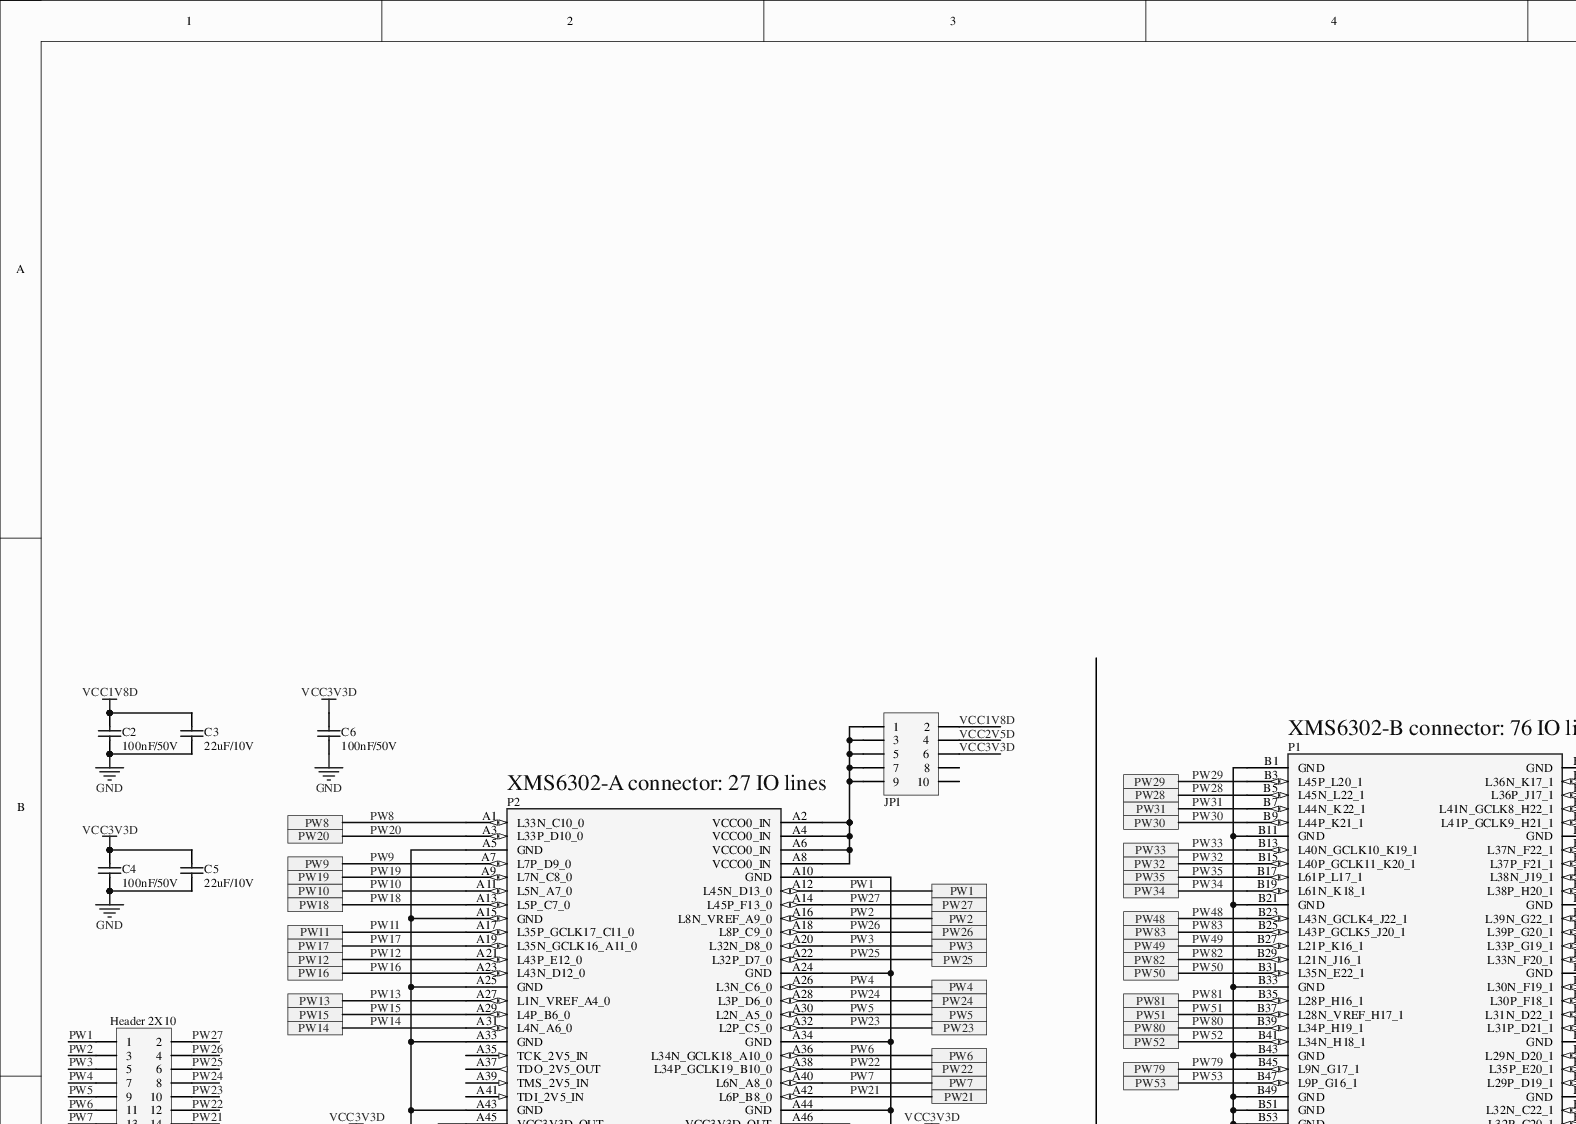
[diagram p0: MISC82195-4.SchDoc, top left]
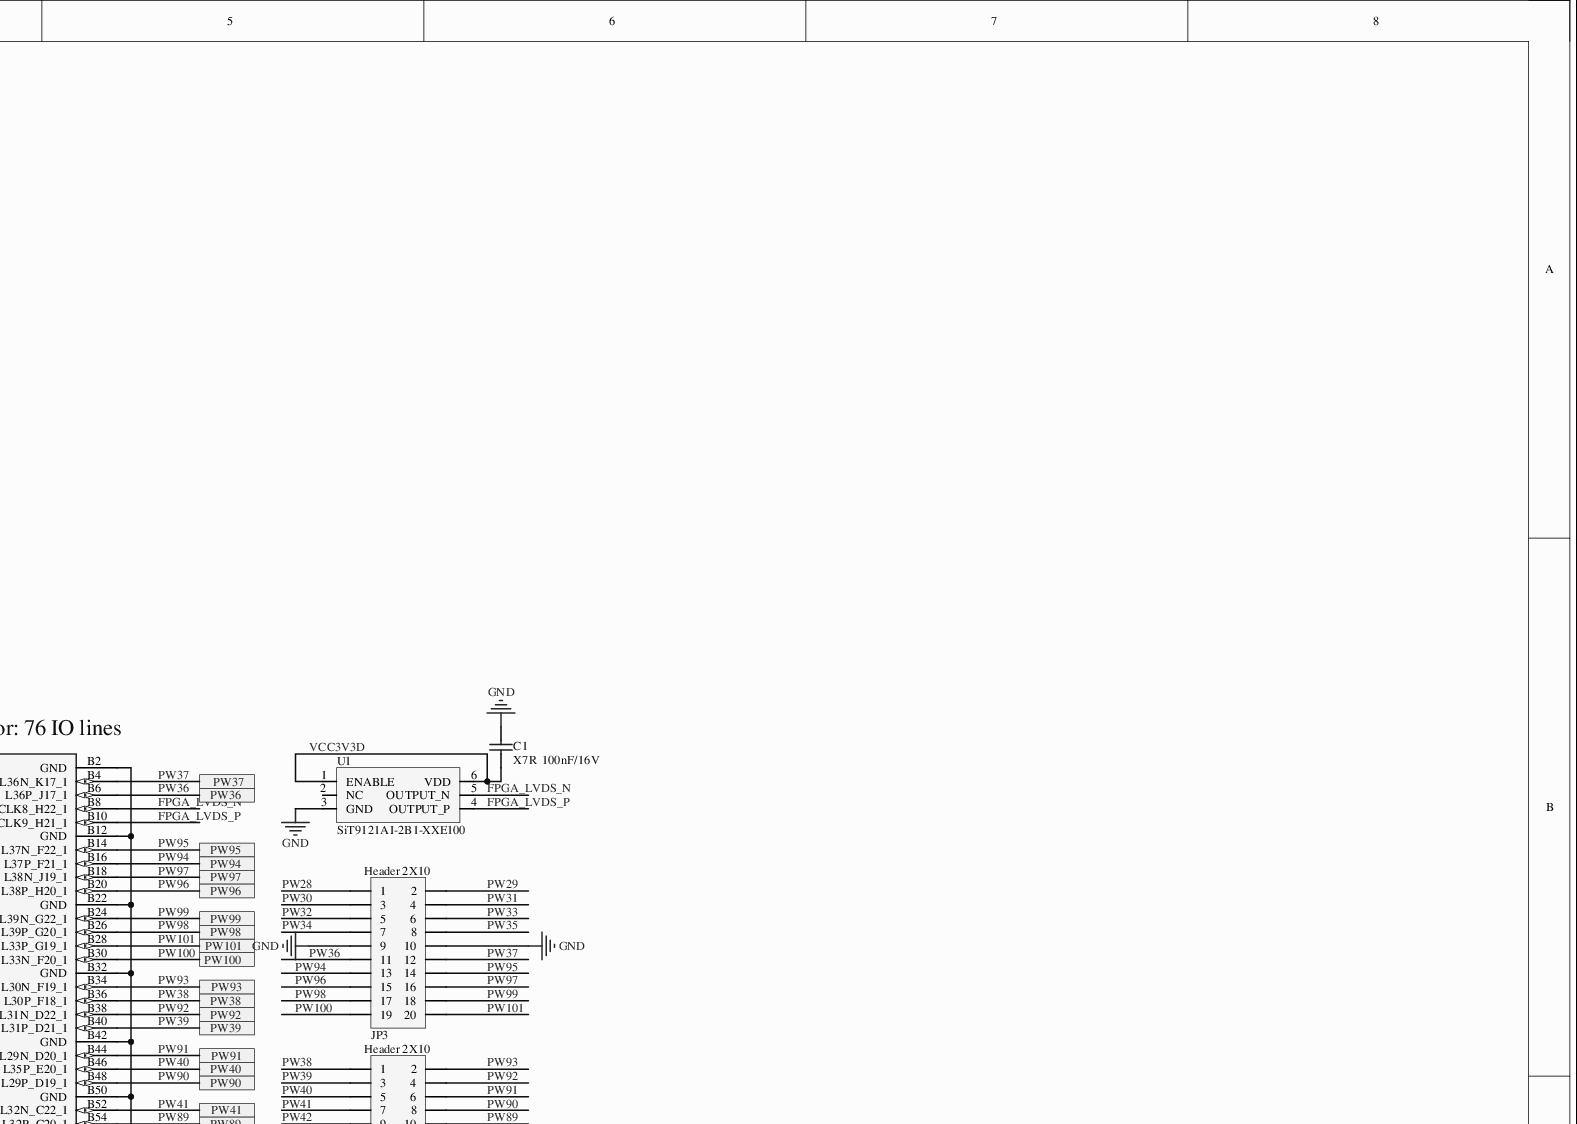
[diagram p1: MISC82195-4.SchDoc, top right]
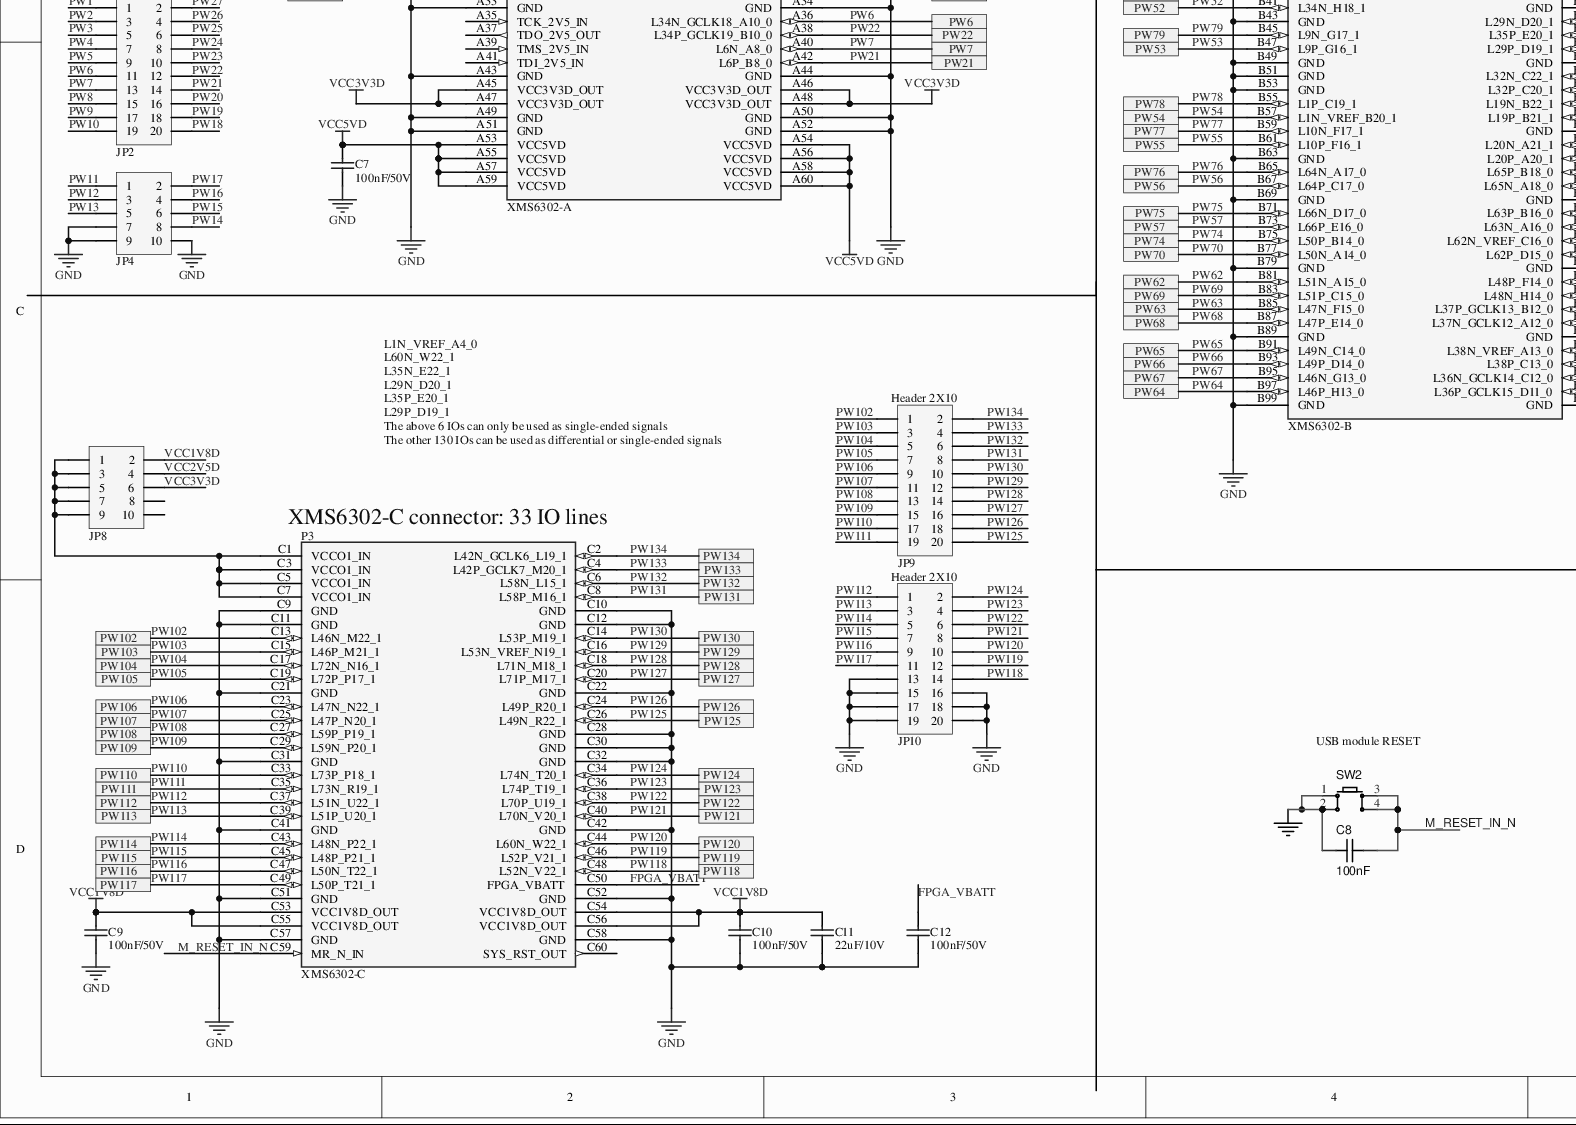
[diagram p2: MISC82195-4.SchDoc, bottom left]
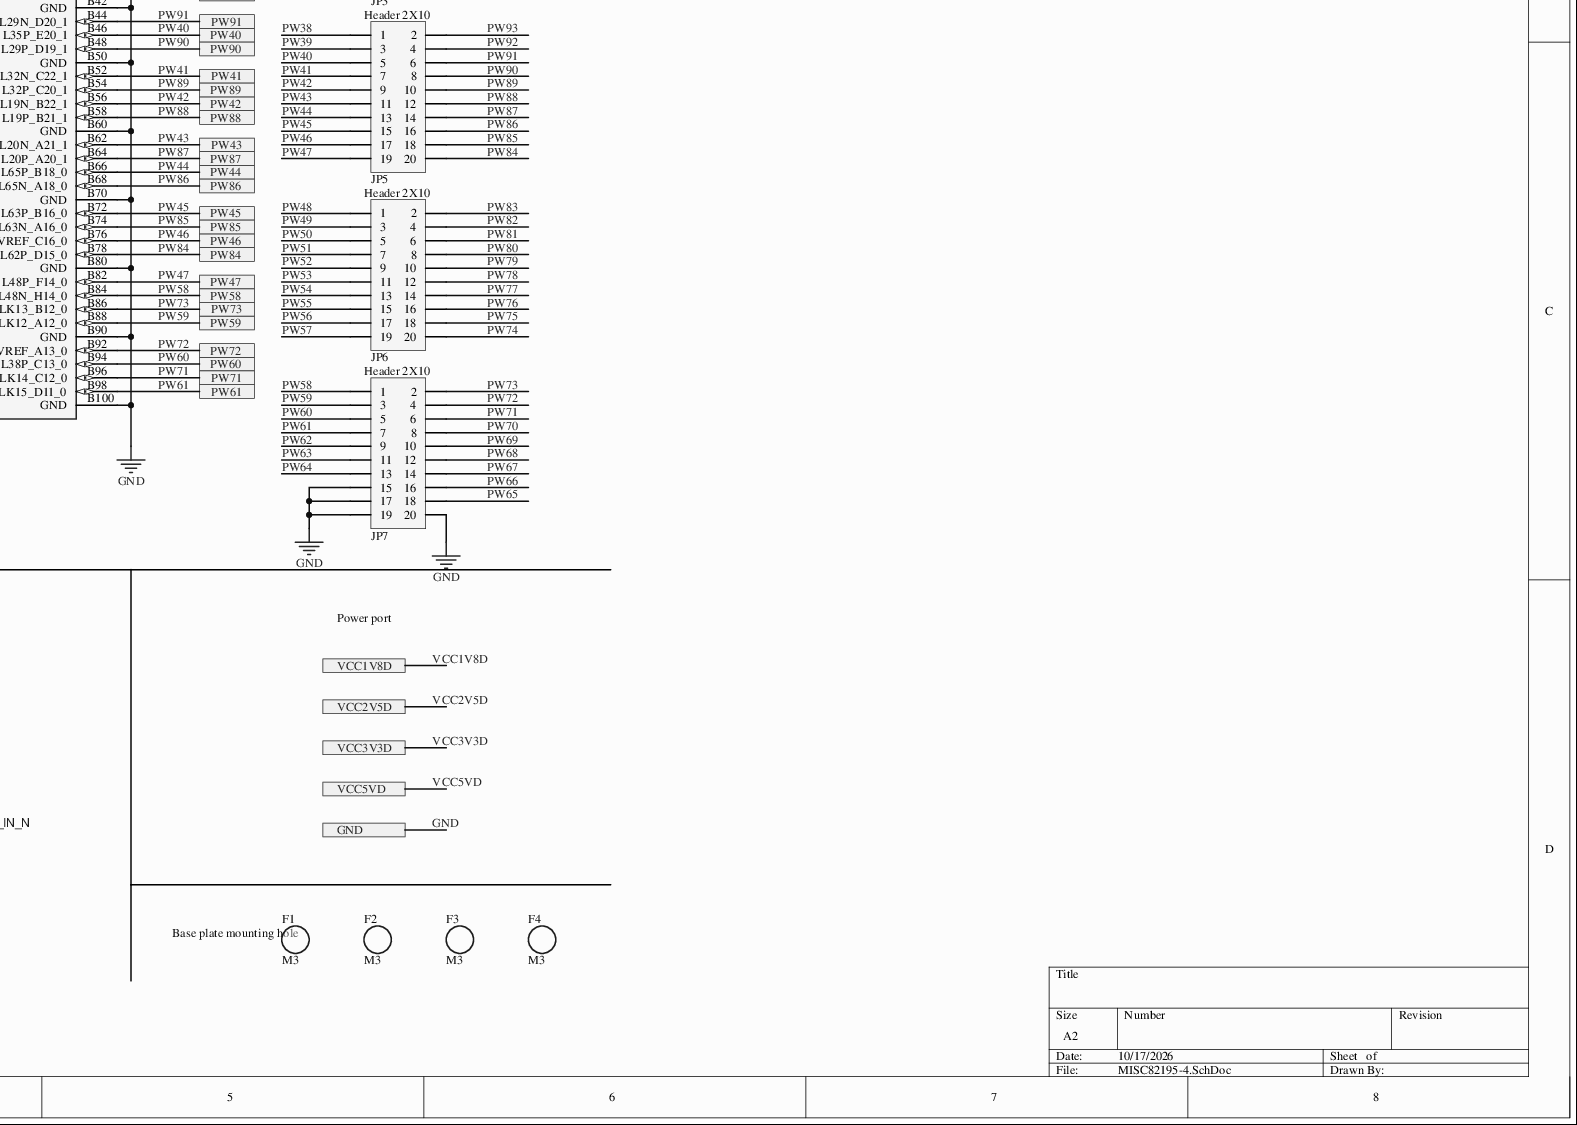
[diagram p3: MISC82195-4.SchDoc, bottom right]
# Altium project MISC82195-8.PrjPcb (part 1 of 2)
3 sheets, 214 parts. Net scope: global (net labels, ports and power ports of the same name join across sheets).
Board file: MISC82195.PcbDoc
Sheets:
  MISC82195-4.SchDoc
  MISC82195-2.SchDoc
  MISC82195-10.SchDoc

## Sheet MISC82195-4.SchDoc
size A2; SheetNumber: 1; SheetTotal: 3

### Parts
C1  X7R  100nF/16V  [C0603]
C2  100nF/50V  [C0603]
C3  22uF/10V  [C0603]
C4  100nF/50V  [C0603]
C5  22uF/10V  [C0603]
C6  100nF/50V  [C0603]
C7  100nF/50V  [C0603]
C8  100nF  [C0603]
C9  100nF/50V  [C0603]
C10  100nF/50V  [C0603]
C11  22uF/10V  [C0603]
C12  100nF/50V  [C0603]
F1  M3  [M3]
F2  M3  [M3]
F3  M3  [M3]
F4  M3  [M3]
JP1  Header 5X2  [HDR2.54-LI-2x5P]  (value not drawn)
JP2  Header 2X10  [HDR2.54-LI-2x10P]
JP3  Header 2X10  [HDR2.54-LI-2x10P]
JP4  Header 5X2  [HDR2.54-LI-2x5P]  (value not drawn)
JP5  Header 2X10  [HDR2.54-LI-2x10P]
JP6  Header 2X10  [HDR2.54-LI-2x10P]
JP7  Header 2X10  [HDR2.54-LI-2x10P]
JP8  Header 5X2  [HDR2.54-LI-2x5P]  (value not drawn)
JP9  Header 2X10  [HDR2.54-LI-2x10P]
JP10  Header 2X10  [HDR2.54-LI-2x10P]
P1  XMS6302-B  [XMS6302-B]
P2  XMS6302-A  [XMS6302-A]
P3  XMS6302-C  [XMS6302-C]
SW2  Key_SMD_6x6x6.5  [SW-SMD_4P-L6.0-W6.0-P4.50-LS9.0-2]  (value not drawn)
U1  SiT9121AI-2B1-XXE100  [3225-6p]

### Ports
GND, PW1, PW2, PW3, PW4, PW5, PW6, PW7, PW8, PW9, PW10, PW11, PW12, PW13, PW14, PW15, PW16, PW17, PW18, PW19, PW20, PW21, PW22, PW23, PW24, PW25, PW26, PW27, PW28, PW29, PW30, PW31, PW32, PW33, PW34, PW35, PW36, PW37, PW38, PW39, PW40, PW41, PW42, PW43, PW44, PW45, PW46, PW47, PW48, PW49, PW50, PW51, PW52, PW53, PW54, PW55, PW56, PW57, PW58, PW59, PW60, PW61, PW62, PW63, PW64, PW65, PW66, PW67, PW68, PW69, PW70, PW71, PW72, PW73, PW74, PW75, PW76, PW77, PW78, PW79, PW80, PW81, PW82, PW83, PW84, PW85, PW86, PW87, PW88, PW89, PW90, PW91, PW92, PW93, PW94, PW95, PW96, PW97, PW98, PW99, PW100, PW101, PW102, PW103, PW104, PW105, PW106, PW107, PW108, PW109, PW110, PW111, PW112, PW113, PW114, PW115, PW116, PW117, PW118, PW119, PW120, PW121, PW122, PW123, PW124, PW125, PW126, PW127, PW128, PW129, PW130, PW131, PW132, PW133, PW134, VCC1V8D, VCC2V5D, VCC3V3D, VCC5VD

### Nets
GND: C1.2 C2.1 C3.1 C4.1 C5.1 C6.1 C7.1 C8.2 C9.1 C10.1 C11.1 C12.2 JP3.9 JP3.10 JP4.7 JP4.9 JP4.10 JP7.15 JP7.17 JP7.19 JP7.20 JP10.13 JP10.15 JP10.16 JP10.17 JP10.18 JP10.19 JP10.20 P1.B1(GND) P1.B2(GND) P1.B11(GND) P1.B12(GND) P1.B21(GND) P1.B22(GND) P1.B32(GND) P1.B33(GND) P1.B42(GND) P1.B43(GND) P1.B49(GND) P1.B50(GND) P1.B51(GND) P1.B53(GND) P1.B60(GND) P1.B63(GND) P1.B69(GND) P1.B70(GND) P1.B79(GND) P1.B80(GND) P1.B89(GND) P1.B90(GND) P1.B99(GND) P1.B100(GND) P2.A5(GND) P2.A10(GND) P2.A15(GND) P2.A24(GND) P2.A25(GND) P2.A33(GND) P2.A34(GND) P2.A43(GND) P2.A44(GND) P2.A49(GND) P2.A50(GND) P2.A51(GND) P2.A52(GND) P3.C9(GND) P3.C10(GND) P3.C11(GND) P3.C12(GND) P3.C21(GND) P3.C22(GND) P3.C28(GND) P3.C30(GND) P3.C31(GND) P3.C32(GND) P3.C41(GND) P3.C42(GND) P3.C51(GND) P3.C52(GND) P3.C57(GND) P3.C58(GND) SW2.1 SW2.2 U1.3(GND) ; port GND
VCC1V8D: C2.2 C3.2 C9.2 C10.2 C11.2 JP1.2 JP8.2 P3.C53(VCC1V8D_OUT) P3.C54(VCC1V8D_OUT) P3.C55(VCC1V8D_OUT) P3.C56(VCC1V8D_OUT) ; port VCC1V8D
VCC3V3D: C1.1 C4.2 C5.2 C6.2 JP1.6 JP8.6 P2.A45(VCC3V3D_OUT) P2.A46(VCC3V3D_OUT) P2.A47(VCC3V3D_OUT) P2.A48(VCC3V3D_OUT) U1.1(ENABLE) U1.6(VDD) ; port VCC3V3D
VCC5VD: C7.2 P2.A53(VCC5VD) P2.A54(VCC5VD) P2.A55(VCC5VD) P2.A56(VCC5VD) P2.A57(VCC5VD) P2.A58(VCC5VD) P2.A59(VCC5VD) P2.A60(VCC5VD) ; port VCC5VD
FPGA_LVDS_N: P1.B8(L41N_GCLK8_H22_1) U1.5(OUTPUT_N)
FPGA_LVDS_P: P1.B10(L41P_GCLK9_H21_1) U1.4(OUTPUT_P)
FPGA_VBATT: C12.1 P3.C50(FPGA_VBATT)
M_RESET_IN_N: C8.1 P3.C59(MR_N_IN) SW2.3 SW2.4
PW1: JP2.1 P2.A12(L45N_D13_0) ; port PW1
PW2: JP2.3 P2.A16(L8N_VREF_A9_0) ; port PW2
PW3: JP2.5 P2.A20(L32N_D8_0) ; port PW3
PW4: JP2.7 P2.A26(L3N_C6_0) ; port PW4  [project net CS_DAC1]
PW5: JP2.9 P2.A30(L2N_A5_0) ; port PW5  [project net CS_DAC2]
PW6: JP2.11 P2.A36(L34N_GCLK18_A10_0) ; port PW6  [project net CS_DAC3]
PW7: JP2.13 P2.A40(L6N_A8_0) ; port PW7
PW8: JP2.15 P2.A1(L33N_C10_0) ; port PW8
PW9: JP2.17 P2.A7(L7P_D9_0) ; port PW9
PW10: JP2.19 P2.A11(L5N_A7_0) ; port PW10
PW11: JP4.1 P2.A17(L35P_GCLK17_C11_0) ; port PW11
PW12: JP4.3 P2.A21(L43P_E12_0) ; port PW12
PW13: JP4.5 P2.A27(L1N_VREF_A4_0) ; port PW13
PW14: JP4.8 P2.A31(L4N_A6_0) ; port PW14
PW15: JP4.6 P2.A29(L4P_B6_0) ; port PW15
PW16: JP4.4 P2.A23(L43N_D12_0) ; port PW16
PW17: JP4.2 P2.A19(L35N_GCLK16_A11_0) ; port PW17
PW18: JP2.20 P2.A13(L5P_C7_0) ; port PW18
PW19: JP2.18 P2.A9(L7N_C8_0) ; port PW19
PW20: JP2.16 P2.A3(L33P_D10_0) ; port PW20
PW21: JP2.14 P2.A42(L6P_B8_0) ; port PW21
PW22: JP2.12 P2.A38(L34P_GCLK19_B10_0) ; port PW22
PW23: JP2.10 P2.A32(L2P_C5_0) ; port PW23
PW24: JP2.8 P2.A28(L3P_D6_0) ; port PW24
PW25: JP2.6 P2.A22(L32P_D7_0) ; port PW25
PW26: JP2.4 P2.A18(L8P_C9_0) ; port PW26
PW27: JP2.2 P2.A14(L45P_F13_0) ; port PW27
PW28: JP3.1 P1.B5(L45N_L22_1) ; port PW28
PW29: JP3.2 P1.B3(L45P_L20_1) ; port PW29
PW30: JP3.3 P1.B9(L44P_K21_1) ; port PW30
PW31: JP3.4 P1.B7(L44N_K22_1) ; port PW31
PW32: JP3.5 P1.B15(L40P_GCLK11_K20_1) ; port PW32
PW33: JP3.6 P1.B13(L40N_GCLK10_K19_1) ; port PW33
PW34: JP3.7 P1.B19(L61N_K18_1) ; port PW34
PW35: JP3.8 P1.B17(L61P_L17_1) ; port PW35
PW36: JP3.11 P1.B6(L36P_J17_1) ; port PW36
PW37: JP3.12 P1.B4(L36N_K17_1) ; port PW37
PW38: JP5.1 P1.B36(L30P_F18_1) ; port PW38
PW39: JP5.3 P1.B40(L31P_D21_1) ; port PW39
PW40: JP5.5 P1.B46(L35P_E20_1) ; port PW40
PW41: JP5.7 P1.B52(L32N_C22_1) ; port PW41
PW42: JP5.9 P1.B56(L19N_B22_1) ; port PW42
PW43: JP5.11 P1.B62(L20N_A21_1) ; port PW43
PW44: JP5.13 P1.B66(L65P_B18_0) ; port PW44
PW45: JP5.15 P1.B72(L63P_B16_0) ; port PW45
PW46: JP5.17 P1.B76(L62N_VREF_C16_0) ; port PW46
PW47: JP5.19 P1.B82(L48P_F14_0) ; port PW47
PW48: JP6.1 P1.B23(L43N_GCLK4_J22_1) ; port PW48
PW49: JP6.3 P1.B27(L21P_K16_1) ; port PW49
PW50: JP6.5 P1.B31(L35N_E22_1) ; port PW50
PW51: JP6.7 P1.B37(L28N_VREF_H17_1) ; port PW51
PW52: JP6.9 P1.B41(L34N_H18_1) ; port PW52
PW53: JP6.11 P1.B47(L9P_G16_1) ; port PW53
PW54: JP6.13 P1.B57(L1N_VREF_B20_1) ; port PW54
PW55: JP6.15 P1.B61(L10P_F16_1) ; port PW55
PW56: JP6.17 P1.B67(L64P_C17_0) ; port PW56
PW57: JP6.19 P1.B73(L66P_E16_0) ; port PW57
PW58: JP7.1 P1.B84(L48N_H14_0) ; port PW58
PW59: JP7.3 P1.B88(L37N_GCLK12_A12_0) ; port PW59
PW60: JP7.5 P1.B94(L38P_C13_0) ; port PW60
PW61: JP7.7 P1.B98(L36P_GCLK15_D11_0) ; port PW61
PW62: JP7.9 P1.B81(L51N_A15_0) ; port PW62
PW63: JP7.11 P1.B85(L47N_F15_0) ; port PW63
PW64: JP7.13 P1.B97(L46P_H13_0) ; port PW64
PW65: JP7.18 P1.B91(L49N_C14_0) ; port PW65
PW66: JP7.16 P1.B93(L49P_D14_0) ; port PW66
PW67: JP7.14 P1.B95(L46N_G13_0) ; port PW67
PW68: JP7.12 P1.B87(L47P_E14_0) ; port PW68
PW69: JP7.10 P1.B83(L51P_C15_0) ; port PW69
PW70: JP7.8 P1.B77(L50N_A14_0) ; port PW70
PW71: JP7.6 P1.B96(L36N_GCLK14_C12_0) ; port PW71
PW72: JP7.4 P1.B92(L38N_VREF_A13_0) ; port PW72
PW73: JP7.2 P1.B86(L37P_GCLK13_B12_0) ; port PW73
PW74: JP6.20 P1.B75(L50P_B14_0) ; port PW74
PW75: JP6.18 P1.B71(L66N_D17_0) ; port PW75
PW76: JP6.16 P1.B65(L64N_A17_0) ; port PW76
PW77: JP6.14 P1.B59(L10N_F17_1) ; port PW77
PW78: JP6.12 P1.B55(L1P_C19_1) ; port PW78
PW79: JP6.10 P1.B45(L9N_G17_1) ; port PW79
PW80: JP6.8 P1.B39(L34P_H19_1) ; port PW80
PW81: JP6.6 P1.B35(L28P_H16_1) ; port PW81
PW82: JP6.4 P1.B29(L21N_J16_1) ; port PW82
PW83: JP6.2 P1.B25(L43P_GCLK5_J20_1) ; port PW83
PW84: JP5.20 P1.B78(L62P_D15_0) ; port PW84
PW85: JP5.18 P1.B74(L63N_A16_0) ; port PW85
PW86: JP5.16 P1.B68(L65N_A18_0) ; port PW86
PW87: JP5.14 P1.B64(L20P_A20_1) ; port PW87
PW88: JP5.12 P1.B58(L19P_B21_1) ; port PW88
PW89: JP5.10 P1.B54(L32P_C20_1) ; port PW89
PW90: JP5.8 P1.B48(L29P_D19_1) ; port PW90
PW91: JP5.6 P1.B44(L29N_D20_1) ; port PW91
PW92: JP5.4 P1.B38(L31N_D22_1) ; port PW92
PW93: JP5.2 P1.B34(L30N_F19_1) ; port PW93  [project net CS_CDAC1]
PW94: JP3.13 P1.B16(L37P_F21_1) ; port PW94
PW95: JP3.14 P1.B14(L37N_F22_1) ; port PW95
PW96: JP3.15 P1.B20(L38P_H20_1) ; port PW96
PW97: JP3.16 P1.B18(L38N_J19_1) ; port PW97
PW98: JP3.17 P1.B26(L39P_G20_1) ; port PW98
PW99: JP3.18 P1.B24(L39N_G22_1) ; port PW99
PW100: JP3.19 P1.B30(L33N_F20_1) ; port PW100
PW101: JP3.20 P1.B28(L33P_G19_1) ; port PW101
PW102: JP9.1 P3.C13(L46N_M22_1) ; port PW102
PW103: JP9.3 P3.C15(L46P_M21_1) ; port PW103
PW104: JP9.5 P3.C17(L72N_N16_1) ; port PW104
PW105: JP9.7 P3.C19(L72P_P17_1) ; port PW105
PW106: JP9.9 P3.C23(L47N_N22_1) ; port PW106
PW107: JP9.11 P3.C25(L47P_N20_1) ; port PW107
PW108: JP9.13 P3.C27(L59P_P19_1) ; port PW108
PW109: JP9.15 P3.C29(L59N_P20_1) ; port PW109
PW110: JP9.17 P3.C33(L73P_P18_1) ; port PW110
PW111: JP9.19 P3.C35(L73N_R19_1) ; port PW111
PW112: JP10.1 P3.C37(L51N_U22_1) ; port PW112
PW113: JP10.3 P3.C39(L51P_U20_1) ; port PW113
PW114: JP10.5 P3.C43(L48N_P22_1) ; port PW114
PW115: JP10.7 P3.C45(L48P_P21_1) ; port PW115
PW116: JP10.9 P3.C47(L50N_T22_1) ; port PW116
PW117: JP10.11 P3.C49(L50P_T21_1) ; port PW117
PW118: JP10.14 P3.C48(L52N_V22_1) ; port PW118
PW119: JP10.12 P3.C46(L52P_V21_1) ; port PW119
PW120: JP10.10 P3.C44(L60N_W22_1) ; port PW120
PW121: JP10.8 P3.C40(L70N_V20_1) ; port PW121
PW122: JP10.6 P3.C38(L70P_U19_1) ; port PW122
PW123: JP10.4 P3.C36(L74P_T19_1) ; port PW123
PW124: JP10.2 P3.C34(L74N_T20_1) ; port PW124
PW125: JP9.20 P3.C26(L49N_R22_1) ; port PW125
PW126: JP9.18 P3.C24(L49P_R20_1) ; port PW126
PW127: JP9.16 P3.C20(L71P_M17_1) ; port PW127
PW128: JP9.14 P3.C18(L71N_M18_1) ; port PW128
PW129: JP9.12 P3.C16(L53N_VREF_N19_1) ; port PW129
PW130: JP9.10 P3.C14(L53P_M19_1) ; port PW130
PW131: JP9.8 P3.C8(L58P_M16_1) ; port PW131
PW132: JP9.6 P3.C6(L58N_L15_1) ; port PW132
PW133: JP9.4 P3.C4(L42P_GCLK7_M20_1) ; port PW133
PW134: JP9.2 P3.C2(L42N_GCLK6_L19_1) ; port PW134
VCC2V5D: JP1.4 JP8.4 ; port VCC2V5D
NetJP1_1: JP1.1 JP1.3 JP1.5 JP1.7 JP1.9 P2.A2(VCCO0_IN) P2.A4(VCCO0_IN) P2.A6(VCCO0_IN) P2.A8(VCCO0_IN)
NetJP8_1: JP8.1 JP8.3 JP8.5 JP8.7 JP8.9 P3.C1(VCCO1_IN) P3.C3(VCCO1_IN) P3.C5(VCCO1_IN) P3.C7(VCCO1_IN)

Not connected (* = marked no-connect by the designer): JP1 8 10; JP8 8 10; P2 A35(TCK_2V5_IN) A37(TDO_2V5_OUT) A39(TMS_2V5_IN) A41(TDI_2V5_IN); P3 C60(SYS_RST_OUT); U1 2(NC)

### Notes on the sheet
- (near P1) XMS6302-B connector: 76 IO lines
- XMS6302-A connector: 27 IO lines
- L1N_VREF_A4_0
- L60N_W22_1
- L35N_E22_1
- L29N_D20_1
- L35P_E20_1
- L29P_D19_1
- The above 6 IOs can only be used as single-ended signals
- The other 130 IOs can be used as differential or single-ended signals
- (near P3) XMS6302-C connector: 33 IO lines
- Power port
- (near SW2) USB module RESET
- (near F1) Base plate mounting hole

### Library data of the parts
C1-C7 C9-C12 = C: SMD capacitor; BOM名称: Non-polar SMD capacitor
C8 = CC0603KRX7R9BB104: Manufacturer: YAGEO(国巨); Add into BOM: yes; Tolerance: ±10%; Voltage Rated: 50V; Temperature Coefficient: X7R; Name: 100nF; Symbol: CC0603KRX7R9BB104; Device: CC0603KRX7R9BB104; Supplier: LCSC; Manufacturer Part: CC0603KRX7R9BB104; Value: 100nF; Supplier Part: C14663; JLCPCB Part Class: Basic library; LCSC Part Name: 100nF ±10% 50V; Supplier Footprint: 0603; Datasheet: https://atta.szlcsc.com/upload/public/pdf/source/20180910/C282072_33301C7F631E79921B82A8DAC6BCC5B3.pdf; Convert to PCB: yes
F1-F4 = M3: Standoff hole; BOM名称: Standoff hole
JP1 JP4 JP8 = Header 5X2: 5*2P connector; BOM名称: 5*2P connector
JP2 JP3 JP5-JP7 JP9 JP10 = Header 10X2: 10*2P connector; BOM名称: 10*2P connector
SW2 = Key_SMD_6x6x6.5: Symbol: Tactile push button; Convert to PCB: yes; Device: Key_SMD_6x6x6.5; Add into BOM: yes; Supplier Footprint: SMD
U1 = SiT9121AI: 100MHz oscillator

## Sheet MISC82195-2.SchDoc
size A3; SheetNumber: 2; SheetTotal: 3
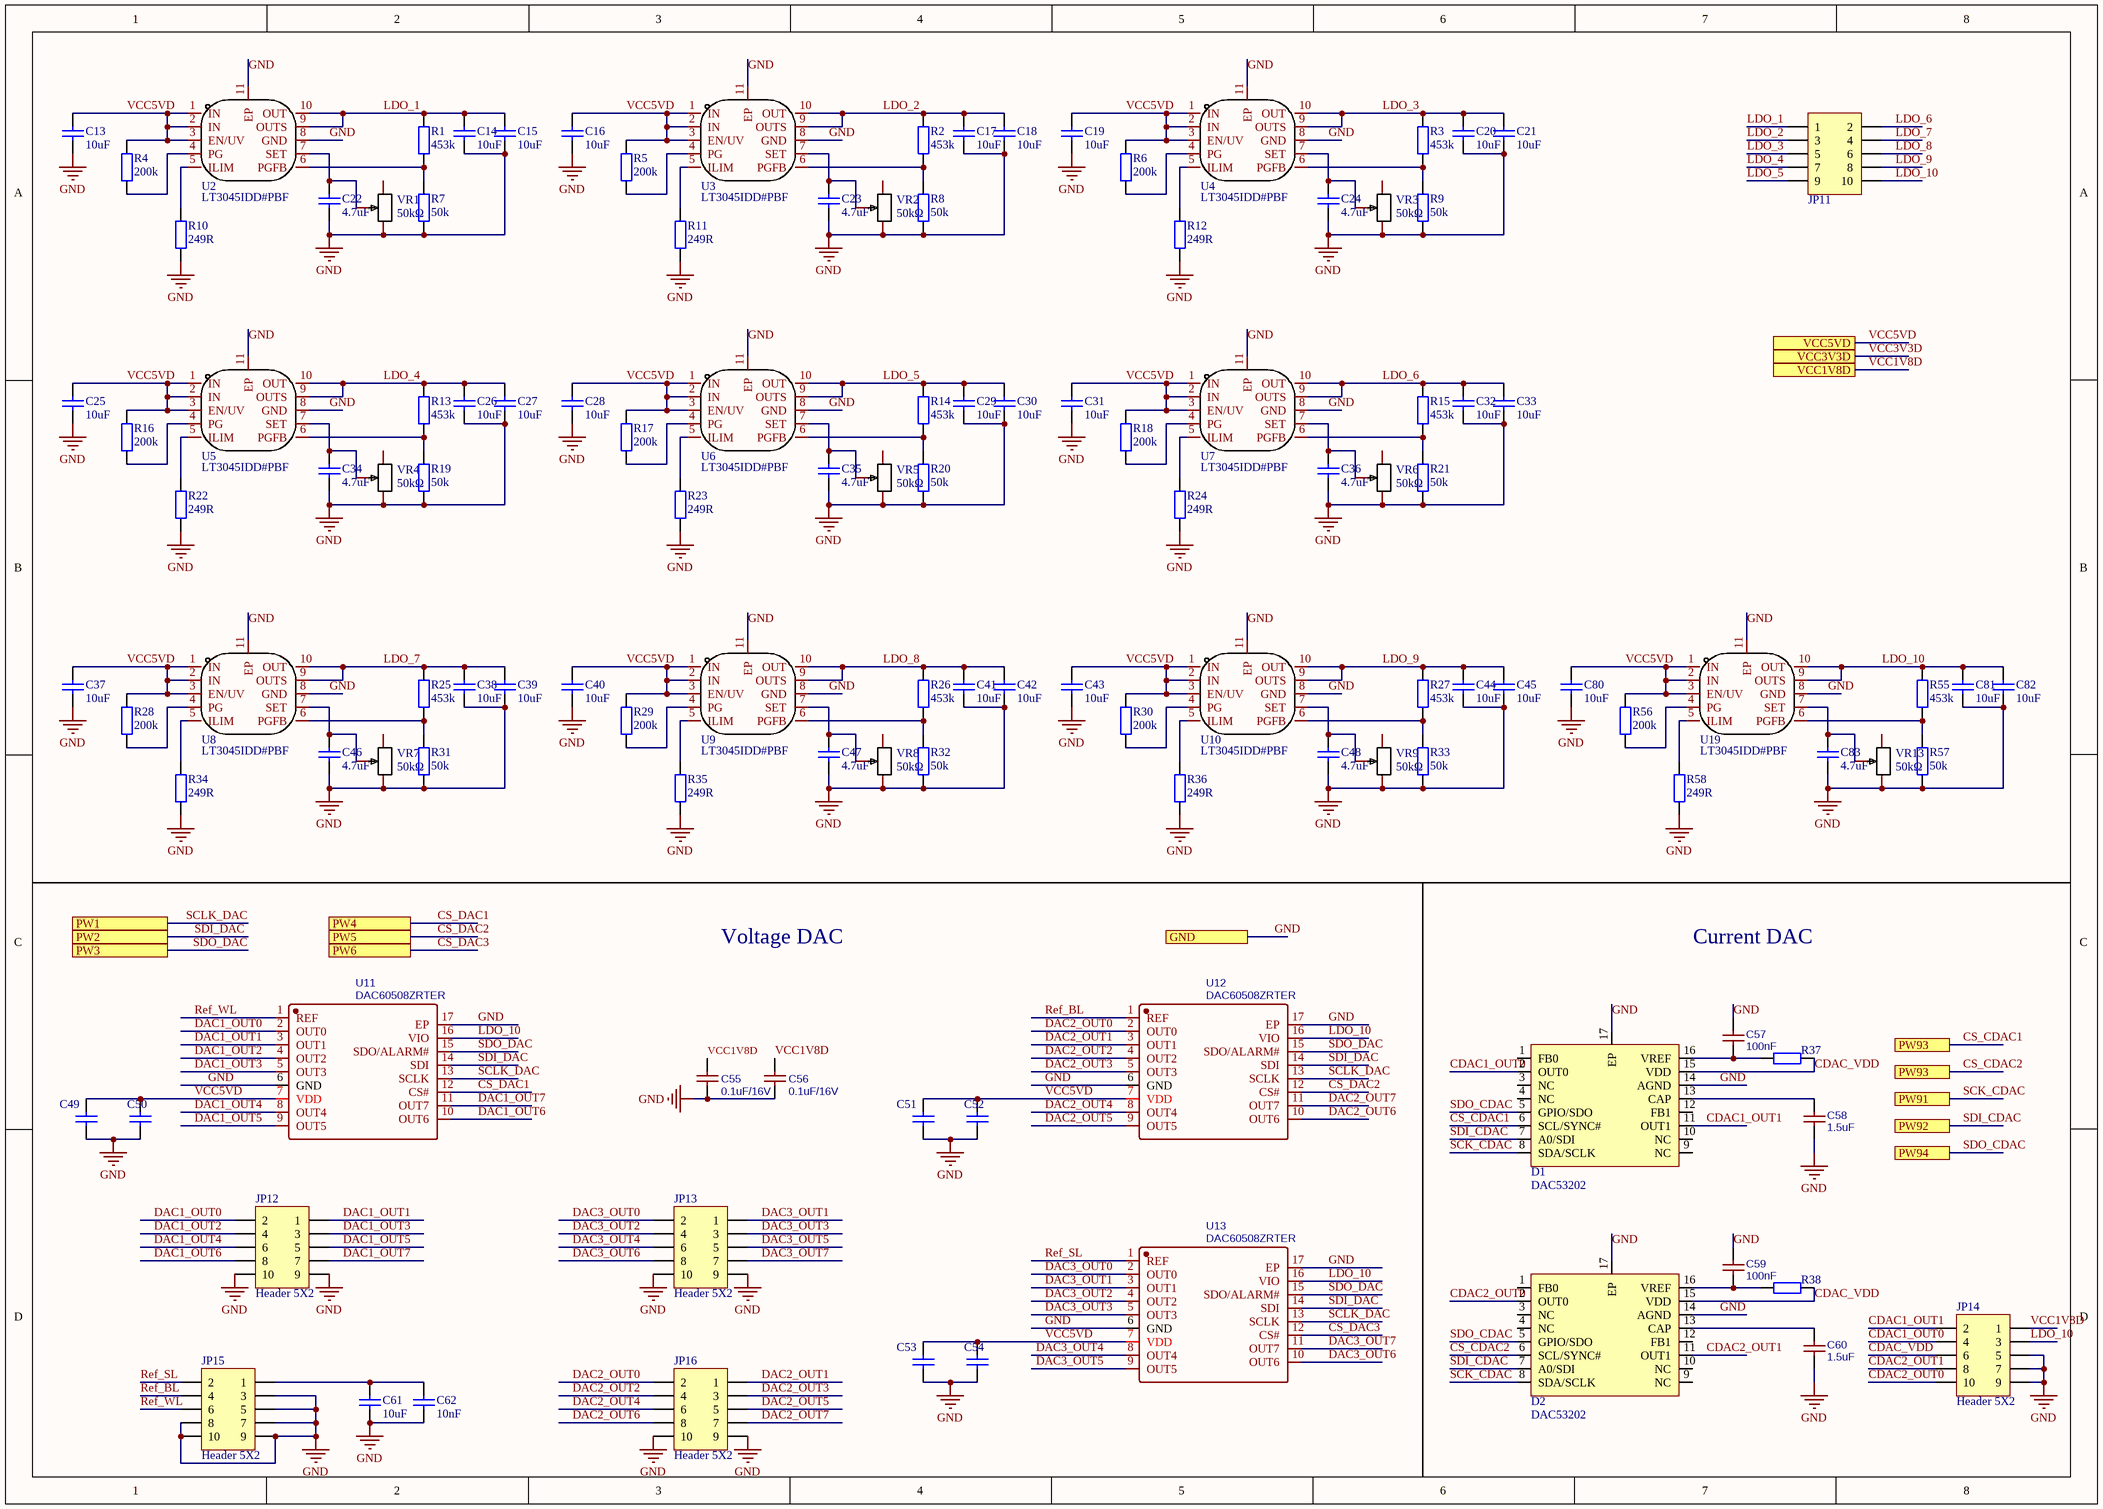
[diagram p4: MISC82195-2.SchDoc]

### Parts
C13  10uF  [C0603]
C14  10uF  [C0603]
C15  10uF  [C0603]
C16  10uF  [C0603]
C17  10uF  [C0603]
C18  10uF  [C0603]
C19  10uF  [C0603]
C20  10uF  [C0603]
C21  10uF  [C0603]
C22  4.7uF  [C0603]
C23  4.7uF  [C0603]
C24  4.7uF  [C0603]
C25  10uF  [C0603]
C26  10uF  [C0603]
C27  10uF  [C0603]
C28  10uF  [C0603]
C29  10uF  [C0603]
C30  10uF  [C0603]
C31  10uF  [C0603]
C32  10uF  [C0603]
C33  10uF  [C0603]
C34  4.7uF  [C0603]
C35  4.7uF  [C0603]
C36  4.7uF  [C0603]
C37  10uF  [C0603]
C38  10uF  [C0603]
C39  10uF  [C0603]
C40  10uF  [C0603]
C41  10uF  [C0603]
C42  10uF  [C0603]
C43  10uF  [C0603]
C44  10uF  [C0603]
C45  10uF  [C0603]
C46  4.7uF  [C0603]
C47  4.7uF  [C0603]
C48  4.7uF  [C0603]
C49  10uF  [C0603]  (value not drawn)
C50  100nF  [C0603]  (value not drawn)
C51  10uF  [C0603]  (value not drawn)
C52  100nF  [C0603]  (value not drawn)
C53  10uF  [C0603]  (value not drawn)
C54  100nF  [C0603]  (value not drawn)
C55  0.1uF/16V  [C0603]
C56  0.1uF/16V  [C0603]
C57  100nF  [C0603]
C58  1.5uF  [C0603]
C59  100nF  [C0603]
C60  1.5uF  [C0603]
C61  10uF  [C0603]
C62  10nF  [C0603]
C80  10uF  [C0603]
C81  10uF  [C0603]
C82  10uF  [C0603]
C83  4.7uF  [C0603]
D1  DAC53202  [WQFN-16(3x3)]
D2  DAC53202  [WQFN-16(3x3)]
JP11  Header 5X2  [HDR2.54-LI-2x5P]  (value not drawn)
JP12  Header 5X2  [HDR2.54-LI-2x5P]
JP13  Header 5X2  [HDR2.54-LI-2x5P]
JP14  Header 5X2  [HDR2.54-LI-2x5P]
JP15  Header 5X2  [HDR2.54-LI-2x5P]
JP16  Header 5X2  [HDR2.54-LI-2x5P]
R1  453k  [R0603]
R2  453k  [R0603]
R3  453k  [R0603]
R4  200k  [R0603]
R5  200k  [R0603]
R6  200k  [R0603]
R7  50k  [R0603]
R8  50k  [R0603]
R9  50k  [R0603]
R10  249R  [R0603]
R11  249R  [R0603]
R12  249R  [R0603]
R13  453k  [R0603]
R14  453k  [R0603]
R15  453k  [R0603]
R16  200k  [R0603]
R17  200k  [R0603]
R18  200k  [R0603]
R19  50k  [R0603]
R20  50k  [R0603]
R21  50k  [R0603]
R22  249R  [R0603]
R23  249R  [R0603]
R24  249R  [R0603]
R25  453k  [R0603]
R26  453k  [R0603]
R27  453k  [R0603]
R28  200k  [R0603]
R29  200k  [R0603]
R30  200k  [R0603]
R31  50k  [R0603]
R32  50k  [R0603]
R33  50k  [R0603]
R34  249R  [R0603]
R35  249R  [R0603]
R36  249R  [R0603]
R37  10K  [R0603]  (value not drawn)
R38  10K  [R0603]  (value not drawn)
R55  453k  [R0603]
R56  200k  [R0603]
R57  50k  [R0603]
R58  249R  [R0603]
U2  LT3045IDD#PBF  [DFN-10_L3.0-W3.0-P0.50-BL-EP-3]
U3  LT3045IDD#PBF  [DFN-10_L3.0-W3.0-P0.50-BL-EP-3]
U4  LT3045IDD#PBF  [DFN-10_L3.0-W3.0-P0.50-BL-EP-3]
U5  LT3045IDD#PBF  [DFN-10_L3.0-W3.0-P0.50-BL-EP-3]
U6  LT3045IDD#PBF  [DFN-10_L3.0-W3.0-P0.50-BL-EP-3]
U7  LT3045IDD#PBF  [DFN-10_L3.0-W3.0-P0.50-BL-EP-3]
U8  LT3045IDD#PBF  [DFN-10_L3.0-W3.0-P0.50-BL-EP-3]
U9  LT3045IDD#PBF  [DFN-10_L3.0-W3.0-P0.50-BL-EP-3]
U10  LT3045IDD#PBF  [DFN-10_L3.0-W3.0-P0.50-BL-EP-3]
U11  DAC60508ZRTER  [WQFN-16_L3.0-W3.0-P0.50-BL-EP0.8]
U12  DAC60508ZRTER  [WQFN-16_L3.0-W3.0-P0.50-BL-EP0.8]
U13  DAC60508ZRTER  [WQFN-16_L3.0-W3.0-P0.50-BL-EP0.8]
U19  LT3045IDD#PBF  [DFN-10_L3.0-W3.0-P0.50-BL-EP-3]
VR1  50kΩ  [RES-ADJ-SMD_3224W]
VR2  50kΩ  [RES-ADJ-SMD_3224W]
VR3  50kΩ  [RES-ADJ-SMD_3224W]
VR4  50kΩ  [RES-ADJ-SMD_3224W]
VR5  50kΩ  [RES-ADJ-SMD_3224W]
VR6  50kΩ  [RES-ADJ-SMD_3224W]
VR7  50kΩ  [RES-ADJ-SMD_3224W]
VR8  50kΩ  [RES-ADJ-SMD_3224W]
VR9  50kΩ  [RES-ADJ-SMD_3224W]
VR13  50kΩ  [RES-ADJ-SMD_3224W]

### Ports
GND, PW1, PW2, PW3, PW4, PW5, PW6, PW91, PW92, PW93, PW94, VCC1V8D, VCC3V3D, VCC5VD

### Nets
GND: C13.1 C14.1 C15.1 C16.1 C17.1 C18.1 C19.1 C20.1 C21.1 C22.1 C23.1 C24.1 C25.1 C26.1 C27.1 C28.1 C29.1 C30.1 C31.1 C32.1 C33.1 C34.1 C35.1 C36.1 C37.1 C38.1 C39.1 C40.1 C41.1 C42.1 C43.1 C44.1 C45.1 C46.1 C47.1 C48.1 C49.1 C50.1 C51.1 C52.1 C53.1 C54.1 C55.1 C56.1 C57.1 C58.2 C59.1 C60.2 C61.1 C62.1 C80.1 C81.1 C82.1 C83.1 D1.14(AGND) D1.17(EP) D2.14(AGND) D2.17(EP) JP12.9 JP12.10 JP13.9 JP13.10 JP14.5 JP14.7 JP14.9 JP15.3 JP15.5 JP15.7 JP15.8 JP15.9 JP15.10 JP16.9 JP16.10 R7.1 R8.1 R9.1 R10.1 R11.1 R12.1 R19.1 R20.1 R21.1 R22.1 R23.1 R24.1 R31.1 R32.1 R33.1 R34.1 R35.1 R36.1 R57.1 R58.1 U2.8(GND) U2.11(EP) U3.8(GND) U3.11(EP) U4.8(GND) U4.11(EP) U5.8(GND) U5.11(EP) U6.8(GND) U6.11(EP) U7.8(GND) U7.11(EP) U8.8(GND) U8.11(EP) U9.8(GND) U9.11(EP) U10.8(GND) U10.11(EP) U11.6(GND) U11.17(EP) U12.6(GND) U12.17(EP) U13.6(GND) U13.17(EP) U19.8(GND) U19.11(EP) VR1.3 VR2.3 VR3.3 VR4.3 VR5.3 VR6.3 VR7.3 VR8.3 VR9.3 VR13.3 ; port GND
VCC1V8D: C55.2 C56.2 JP14.1 ; port VCC1V8D
VCC5VD: C13.2 C16.2 C19.2 C25.2 C28.2 C31.2 C37.2 C40.2 C43.2 C49.2 C50.2 C51.2 C52.2 C53.2 C54.2 C80.2 R4.2 R5.2 R6.2 R16.2 R17.2 R18.2 R28.2 R29.2 R30.2 R56.2 U2.1(IN) U2.2(IN) U2.3(EN/UV) U3.1(IN) U3.2(IN) U3.3(EN/UV) U4.1(IN) U4.2(IN) U4.3(EN/UV) U5.1(IN) U5.2(IN) U5.3(EN/UV) U6.1(IN) U6.2(IN) U6.3(EN/UV) U7.1(IN) U7.2(IN) U7.3(EN/UV) U8.1(IN) U8.2(IN) U8.3(EN/UV) U9.1(IN) U9.2(IN) U9.3(EN/UV) U10.1(IN) U10.2(IN) U10.3(EN/UV) U11.7(VDD) U12.7(VDD) U13.7(VDD) U19.1(IN) U19.2(IN) U19.3(EN/UV) ; port VCC5VD
CDAC1_OUT0: D1.2(OUT0) JP14.4
CDAC1_OUT1: D1.11(OUT1) JP14.2
CDAC2_OUT0: D2.2(OUT0) JP14.10
CDAC2_OUT1: D2.11(OUT1) JP14.8
CDAC_VDD: D1.15(VDD) D2.15(VDD) JP14.6 R37.2 R38.2
CS_CDAC1: D1.6(SCL/SYNC#) D2.6(SCL/SYNC#) ; port PW93  [also labelled CS_CDAC2]
CS_DAC1: U11.12(CS#) ; port PW4
CS_DAC2: U12.12(CS#) ; port PW5
CS_DAC3: U13.12(CS#) ; port PW6
DAC1_OUT0: JP12.2 U11.2(OUT0)
DAC1_OUT1: JP12.1 U11.3(OUT1)
DAC1_OUT2: JP12.4 U11.4(OUT2)
DAC1_OUT3: JP12.3 U11.5(OUT3)
DAC1_OUT4: JP12.6 U11.8(OUT4)
DAC1_OUT5: JP12.5 U11.9(OUT5)
DAC1_OUT6: JP12.8 U11.10(OUT6)
DAC1_OUT7: JP12.7 U11.11(OUT7)
DAC2_OUT0: JP16.2 U12.2(OUT0)
DAC2_OUT1: JP16.1 U12.3(OUT1)
DAC2_OUT2: JP16.4 U12.4(OUT2)
DAC2_OUT3: JP16.3 U12.5(OUT3)
DAC2_OUT4: JP16.6 U12.8(OUT4)
DAC2_OUT5: JP16.5 U12.9(OUT5)
DAC2_OUT6: JP16.8 U12.10(OUT6)
DAC2_OUT7: JP16.7 U12.11(OUT7)
DAC3_OUT0: JP13.2 U13.2(OUT0)
DAC3_OUT1: JP13.1 U13.3(OUT1)
DAC3_OUT2: JP13.4 U13.4(OUT2)
DAC3_OUT3: JP13.3 U13.5(OUT3)
DAC3_OUT4: JP13.6 U13.8(OUT4)
DAC3_OUT5: JP13.5 U13.9(OUT5)
DAC3_OUT6: JP13.8 U13.10(OUT6)
DAC3_OUT7: JP13.7 U13.11(OUT7)
LDO_1: C14.2 C15.2 JP11.1 R1.2 U2.9(OUTS) U2.10(OUT)
LDO_2: C17.2 C18.2 JP11.3 R2.2 U3.9(OUTS) U3.10(OUT)
LDO_3: C20.2 C21.2 JP11.5 R3.2 U4.9(OUTS) U4.10(OUT)
LDO_4: C26.2 C27.2 JP11.7 R13.2 U5.9(OUTS) U5.10(OUT)
LDO_5: C29.2 C30.2 JP11.9 R14.2 U6.9(OUTS) U6.10(OUT)
LDO_6: C32.2 C33.2 JP11.2 R15.2 U7.9(OUTS) U7.10(OUT)
LDO_7: C38.2 C39.2 JP11.4 R25.2 U8.9(OUTS) U8.10(OUT)
LDO_8: C41.2 C42.2 JP11.6 R26.2 U9.9(OUTS) U9.10(OUT)
LDO_9: C44.2 C45.2 JP11.8 R27.2 U10.9(OUTS) U10.10(OUT)
LDO_10: C81.2 C82.2 JP11.10 JP14.3 R55.2 U11.16(VIO) U12.16(VIO) U13.16(VIO) U19.9(OUTS) U19.10(OUT)
Ref_BL: JP15.4 U12.1(REF)
Ref_SL: JP15.2 U13.1(REF)
Ref_WL: JP15.6 U11.1(REF)
SCK_CDAC: D1.8(SDA/SCLK) D2.8(SDA/SCLK) ; port PW91  [project net PW91]
SCLK_DAC: U11.13(SCLK) U12.13(SCLK) U13.13(SCLK) ; port PW1  [project net PW1]
SDI_CDAC: D1.7(A0/SDI) D2.7(A0/SDI) ; port PW92  [project net PW92]
SDI_DAC: U11.14(SDI) U12.14(SDI) U13.14(SDI) ; port PW2  [project net PW2]
SDO_CDAC: D1.5(GPIO/SDO) D2.5(GPIO/SDO) ; port PW94  [project net PW94]
SDO_DAC: U11.15(SDO/ALARM#) U12.15(SDO/ALARM#) U13.15(SDO/ALARM#) ; port PW3  [project net PW3]
NetC22_2: C22.2 U2.7(SET) VR1.2
NetC23_2: C23.2 U3.7(SET) VR2.2
NetC24_2: C24.2 U4.7(SET) VR3.2
NetC34_2: C34.2 U5.7(SET) VR4.2
NetC35_2: C35.2 U6.7(SET) VR5.2
NetC36_2: C36.2 U7.7(SET) VR6.2
NetC46_2: C46.2 U8.7(SET) VR7.2
NetC47_2: C47.2 U9.7(SET) VR8.2
NetC48_2: C48.2 U10.7(SET) VR9.2
NetC57_2: C57.2 D1.16(VREF) R37.1
NetC58_1: C58.1 D1.13(CAP)
NetC59_2: C59.2 D2.16(VREF) R38.1
NetC60_1: C60.1 D2.13(CAP)
NetC61_2: C61.2 C62.2 JP15.1
NetC83_2: C83.2 U19.7(SET) VR13.2
NetR1_1: R1.1 R7.2 U2.6(PGFB)
NetR2_1: R2.1 R8.2 U3.6(PGFB)
NetR3_1: R3.1 R9.2 U4.6(PGFB)
NetR4_1: R4.1 U2.4(PG)
NetR5_1: R5.1 U3.4(PG)
NetR6_1: R6.1 U4.4(PG)
NetR10_2: R10.2 U2.5(ILIM)
NetR11_2: R11.2 U3.5(ILIM)
NetR12_2: R12.2 U4.5(ILIM)
NetR13_1: R13.1 R19.2 U5.6(PGFB)
NetR14_1: R14.1 R20.2 U6.6(PGFB)
NetR15_1: R15.1 R21.2 U7.6(PGFB)
NetR16_1: R16.1 U5.4(PG)
NetR17_1: R17.1 U6.4(PG)
NetR18_1: R18.1 U7.4(PG)
NetR22_2: R22.2 U5.5(ILIM)
NetR23_2: R23.2 U6.5(ILIM)
NetR24_2: R24.2 U7.5(ILIM)
NetR25_1: R25.1 R31.2 U8.6(PGFB)
NetR26_1: R26.1 R32.2 U9.6(PGFB)
NetR27_1: R27.1 R33.2 U10.6(PGFB)
NetR28_1: R28.1 U8.4(PG)
NetR29_1: R29.1 U9.4(PG)
NetR30_1: R30.1 U10.4(PG)
NetR34_2: R34.2 U8.5(ILIM)
NetR35_2: R35.2 U9.5(ILIM)
NetR36_2: R36.2 U10.5(ILIM)
NetR55_1: R55.1 R57.2 U19.6(PGFB)
NetR56_1: R56.1 U19.4(PG)
NetR58_2: R58.2 U19.5(ILIM)

Not connected (* = marked no-connect by the designer): D1 1(FB0) 3(NC) 4(NC) 9(NC) 10(NC) 12(FB1); D2 1(FB0) 3(NC) 4(NC) 9(NC) 10(NC) 12(FB1); VR1 1; VR2 1; VR3 1; VR4 1; VR5 1; VR6 1; VR7 1; VR8 1; VR9 1; VR13 1

### Notes on the sheet
- Voltage DAC
- Current DAC

### Library data of the parts
C13-C54 C61 C62 C80-C83 = C: as C1 on sheet MISC82195-4
C55 C56 = 10nF: Manufacturer Part: CC0603KRX7R9BB103; nameAlias: Value; Supplier: LCSC; Supplier Part: C100042; JLCPCB Part Class: Extended Part; spicePre: C; spiceSymbolName: CC0603KRX7R9BB103
C57-C60 = 1uF: Manufacturer Part: CL10A105KB8NNNC; nameAlias: Value; Supplier: LCSC; Supplier Part: C15849; JLCPCB Part Class: Basic Part; spicePre: C; spiceSymbolName: CL10A105KB8NNNC
JP11-JP16 = Header 5X2: 5*2P connector; BOM名称: 5*2P connector
R1-R38 R55-R58 = R: SMD resistor; BOM名称: SMD resistor
U2-U10 U19 = LT3045IDD#PBF: Manufacturer: ADI(亚德诺); Add into BOM: yes; Output Type: Adjustable; Maximum Input Voltage: 20V; Output Voltage: 0V~15V; MAX Output Current: 500mA; Dropout Voltage: 450mV@(500mA); standby current: 20uA; Output Polarity: Positive; Number of Outputs: 1; Name: LT3045IDD#PBF; Symbol: LT3045IDD#PBF; Device: LT3045IDD#PBF; LCSC Part Name: LT3045IDD#PBF; Supplier Part: C580013; Manufacturer Part: LT3045IDD#PBF; Supplier Footprint: DFN-10-EP(3x3); JLCPCB Part Class: Extended library; Datasheet: https://atta.szlcsc.com/upload/public/pdf/source/20200416/C514420_E440C492D6C74EAE6AB301243586F696.pdf; Supplier: LCSC; Convert to PCB: yes; Operating Temperature: -40℃~+125℃@(Tj)
U11-U13 = DAC60508ZRTER: Contributor: LCSC; Supplier: LCSC; Supplier Part: C2679476; Manufacturer Part: DAC60508ZRTER; JLCPCB Part Class: Extended Part; spicePre: U; spiceSymbolName: DAC60508ZRTER
VR1-VR9 VR13 = 3224W-1-503E: Manufacturer: BOURNS; Resistance: 50K; Add into BOM: yes; Tolerance: ±10%; Power(Watts): 250mW; Temperature Coefficient: ±100ppm/℃; Turns: 12; Name: 50kΩ; Symbol: 3224W-1-503E; Device: 3224W-1-503E; Supplier: LCSC; Manufacturer Part: 3224W-1-503E; Supplier Part: C48484; Value: 50kΩ; JLCPCB Part Class: Extended library; LCSC Part Name: 50kΩ ±10%; Supplier Footprint: SMD; Datasheet: https://atta.szlcsc.com/upload/public/pdf/source/20160830/1472551532733.pdf; Convert to PCB: yes